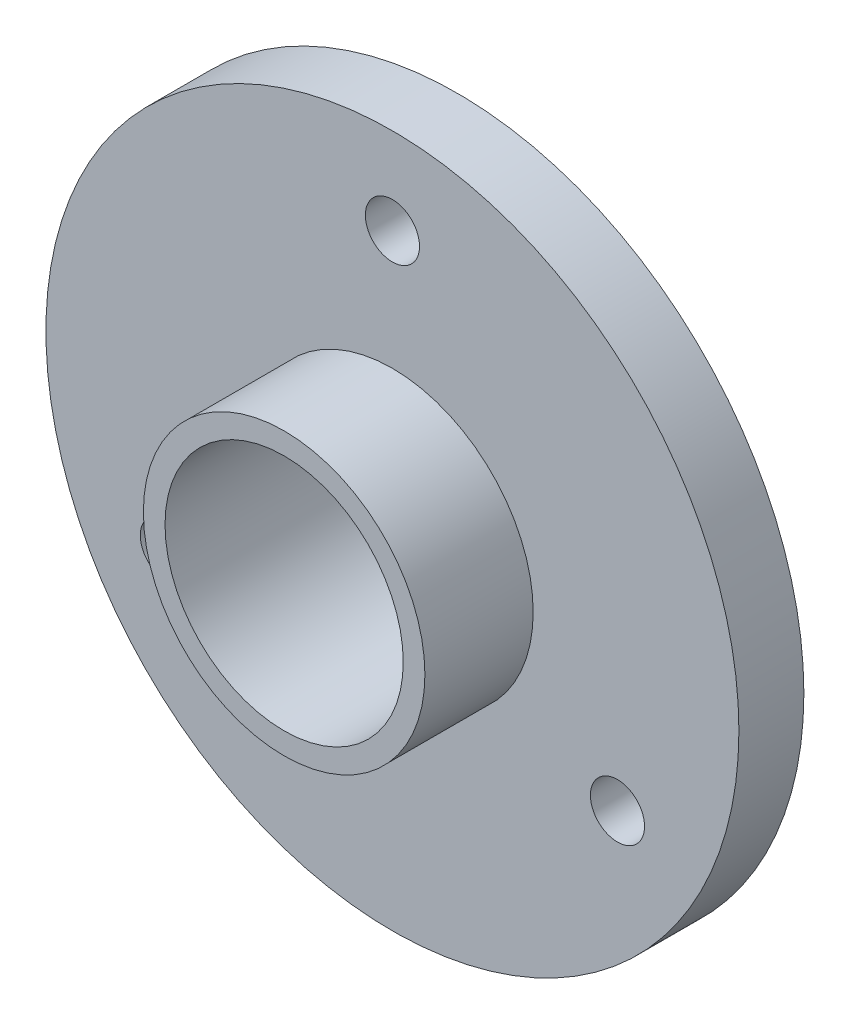
from build123d import *

# Parameters (mm, degrees)
SKETCH1_R             = 16
BOSS_EXTRUDE1_DEPTH   = 3
SKETCH2_R             = 6.5
BOSS_EXTRUDE2_DEPTH   = 5
SKETCH3_R             = 5.5
CUT_EXTRUDE1_DEPTH    = 22
SKETCH4_R             = 1
CUT_EXTRUDE2_DEPTH    = 10
M3_TAPPED_HOLE1_D     = 2.5
M3_TAPPED_HOLE1_DEPTH = 8


with BuildPart() as part:
    # Sketch1 → Boss-Extrude1 (new body)
    with BuildSketch(Plane.XY):
        Circle(SKETCH1_R)
    extrude(amount=BOSS_EXTRUDE1_DEPTH)

    # Sketch2 → Boss-Extrude2 (add)
    with BuildSketch(Plane.XY.offset(3)):
        Circle(SKETCH2_R)
    extrude(amount=BOSS_EXTRUDE2_DEPTH)

    # Sketch3 → Cut-Extrude1 (cut)
    with BuildSketch(Plane(origin=(0, 0, 0), x_dir=(-1, 0, 0), z_dir=(0, 0, -1))):
        Circle(SKETCH3_R)
    extrude(amount=-CUT_EXTRUDE1_DEPTH, mode=Mode.SUBTRACT)

    # Sketch4 → Cut-Extrude2 (cut)
    with BuildSketch(Plane(origin=(0, 0, 0), x_dir=(-1, 0, 0), z_dir=(0, 0, -1))):
        with Locations((0, 12)):
            Circle(SKETCH4_R)
        with Locations((10.392304845, -6)):
            Circle(SKETCH4_R)
        with Locations((-10.392304845, -6)):
            Circle(SKETCH4_R)
    extrude(amount=-CUT_EXTRUDE2_DEPTH, mode=Mode.SUBTRACT)

    # M3 Tapped Hole1
    with Locations(Plane(origin=(0, 0, 0), x_dir=(-1, 0, 0), z_dir=(0, 0, -1))):
        with Locations((0, 12), (10.392304845, -6), (-10.392304845, -6)):
            Hole(M3_TAPPED_HOLE1_D / 2, depth=M3_TAPPED_HOLE1_DEPTH)


solid = part.part
